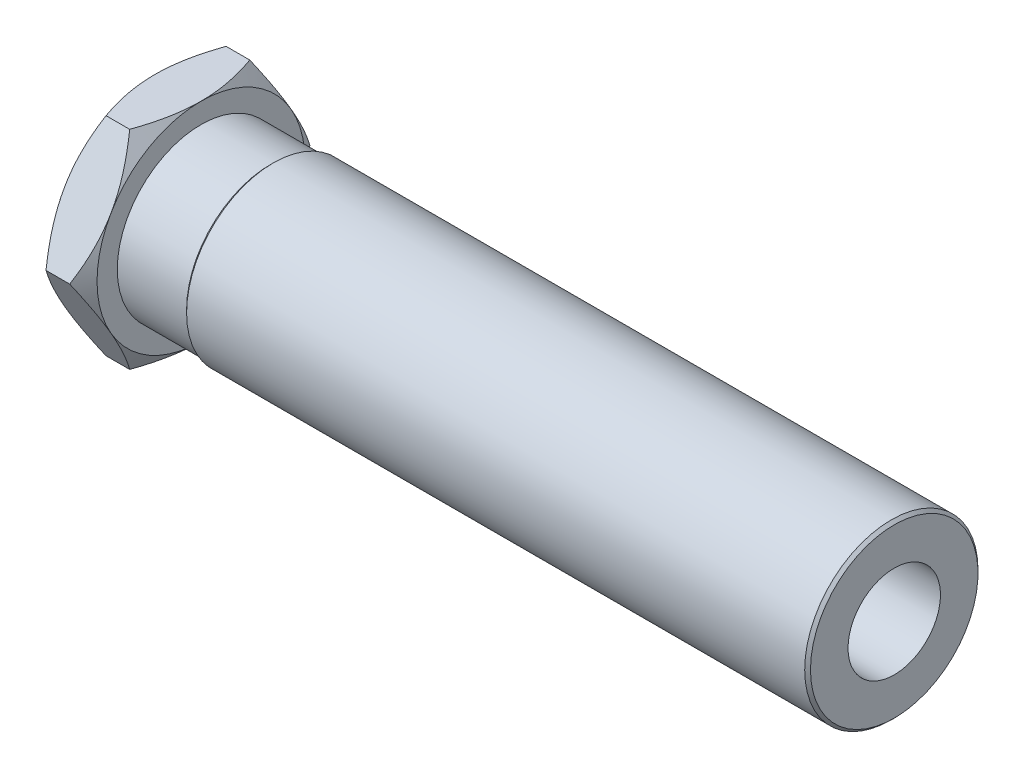
SolidWorks part; units mm, degrees
ref_plane "前视基准面" through (0, 0, 0) normal (0, 0, 1) x (1, 0, 0)
ref_plane "上视基准面" through (0, 0, 0) normal (0, 1, 0) x (1, 0, 0)
ref_plane "右视基准面" through (0, 0, 0) normal (1, 0, 0) x (0, 0, -1)
sketch "草图1" plane through (0, 0, 0) normal (0, 0, 1) x (1, 0, 0)
  line L0 (0, 0) -> (120, 0) construction
  line L1 (120, 0) -> (120, 14.5)
  line L2 (120, 14.5) -> (119.5, 15)
  line L3 (119.5, 15) -> (12.5, 15)
  line L4 (12.5, 15) -> (12, 14.5)
  line L5 (12, 14.5) -> (0, 14.5)
  line L6 (0, 0) -> (0, 14.5)
  line L7 (0, 14.5) -> (0, 18) construction
  line L8 (0, 18) -> (-8, 18)
  line L9 (-8, 18) -> (-8, 0) construction
  line L10 (-8, 0) -> (0, 0) construction
  line L11 (120, 11.5) -> (-8, 11.5)
  dimension "D111" = 0.5
  dimension "D2" = 12
  dimension "D1111" = 135
  dimension "D3111" = 135
  dimension "M" = 30
  dimension "L" = 120
  dimension "T" = 8
  dimension "B" = 36
  dimension "d" = 23
sketch "草图2" plane through (0, 0, 0) normal (0, 0, 1) x (1, 0, 0)
  line L0 (0, 0) -> (120, 0) construction
  line L1 (120, 0) -> (120, 14.5) construction
  line L2 (120, 14.5) -> (119.5, 15) construction
  line L3 (119.5, 15) -> (12.5, 15) construction
  line L4 (12.5, 15) -> (12, 14.5) construction
  line L5 (12, 14.5) -> (0, 14.5) construction
  line L6 (0, 0) -> (0, 14.5) construction
  line L7 (0, 0) -> (120, 0)
  line L8 (120, 0) -> (120, 14.5)
  line L9 (120, 14.5) -> (119.5, 15)
  line L10 (119.5, 15) -> (12.5, 15)
  line L11 (12.5, 15) -> (12, 14.5)
  line L12 (12, 14.5) -> (0, 14.5)
  line L13 (0, 0) -> (0, 14.5)
revolve "旋转1" add sketch "草图2" angle 360 about L7
cosmetic thread "装饰螺纹线1" parameters "D2"=25.5
sketch "螺栓草图1" plane through (0, -0.9101, 0.3973) normal (-1, 0, 0) x (0, 0, 1)
  line L1 (-21.1819, 0.9101) -> (-10.7896, -17.0899)
  line L2 (-10.7896, -17.0899) -> (9.995, -17.0899)
  line L3 (9.995, -17.0899) -> (20.3873, 0.9101)
  line L4 (20.3873, 0.9101) -> (9.995, 18.9101)
  line L5 (9.995, 18.9101) -> (-10.7896, 18.9101)
  line L6 (-10.7896, 18.9101) -> (-21.1819, 0.9101)
  circle A0 centre (-0.3973, 0.9101) radius 18 construction
  dimension "D1" = 36
extrude "拉伸-螺栓" add sketch "螺栓草图1" along normal blind 8
sketch "螺栓草图2" plane through (-8, 0, 0) normal (-1, 0, 0) x (0, 0, 1)
  circle A0 centre (0, 0) radius 18 construction
  circle A1 centre (0, 0) radius 18
  circle A2 centre (0, 0) radius 23.58
  dimension "D1" = 47.16
extrude "切除-螺栓" cut sketch "螺栓草图2" against normal up to vertex (8 mm away) draft 55 up to point (0, 0, 20.7846)
sketch "草图5" plane through (0, 0, 0) normal (1, 0, 0) x (0, 0, -1)
  line L0 (10.3923, 18) -> (20.7846, 0) construction
  line L1 (18, 0) -> (20.7846, 0) construction
  line L2 (20.7846, 0) -> (23.5692, 0) construction
  circle A0 centre (0, 0) radius 18
  circle A1 centre (0, 0) radius 23.5692
extrude "切除-拉伸2" cut sketch "草图5" against normal up to vertex (6.0502 mm away) draft 55 up to point (-6.0502, 0, 20.7846)
sketch "草图6" plane through (0, 0, 0) normal (0, 0, 1) x (1, 0, 0)
  line L0 (0, 0) -> (120, 0) construction
  line L1 (-8, 0) -> (0, 0) construction
  line L5 (0, 0) -> (120, 0)
  line L6 (-8, 0) -> (0, 0)
  line L7 (-8, 8) -> (-8, 0)
  line L8 (120, 8) -> (-8, 8)
  line L9 (120, 0) -> (120, 8)
  line L10 (120, -14.5) -> (120, 14.5) construction
  dimension "D1" = 8
  dimension "D2" = 8
  dimension "D3" = 128
revolve "切除-旋转1" cut sketch "草图6" angle 360 about L5
